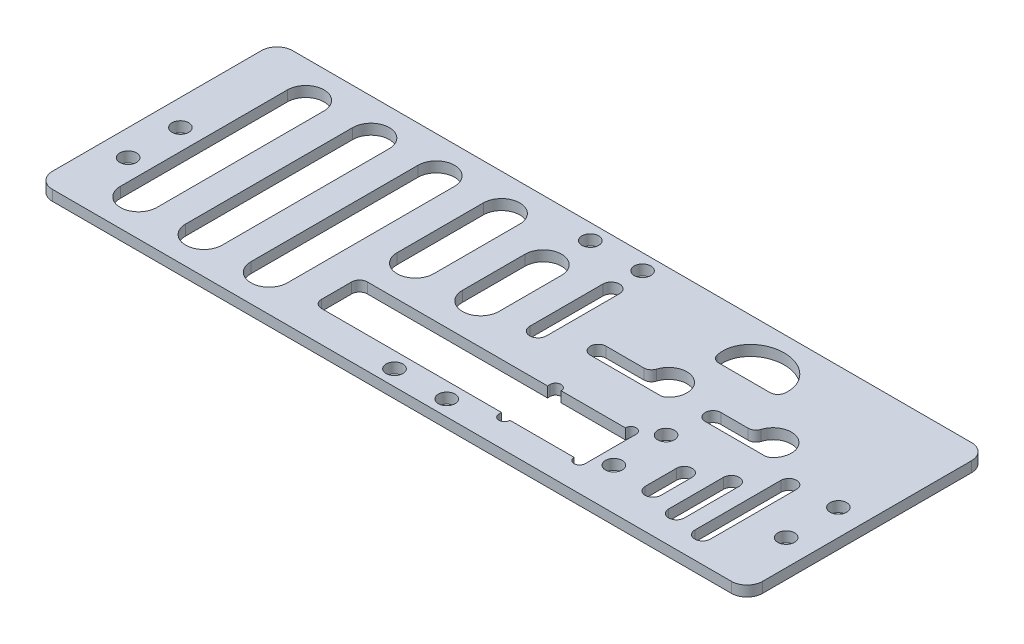
from build123d import *

# Parameters (mm, degrees)
SKETCH_1_W          = 136
SKETCH_1_H          = 46
SKETCH_1_R          = 1.6
EXTRUDE_1_DEPTH     = 2
CUT_EXTRUDE_1_DEPTH = 72.812255222
FILLET_R1_5_R       = 1.5
FILLET_R3_R         = 3


with BuildPart() as part:
    # 草图1 → 凸台-拉伸1 (new body)
    with BuildSketch(Plane(origin=(0, 0, 0), x_dir=(1, 0, 0), z_dir=(0, 1, 0))):
        Rectangle(SKETCH_1_W, SKETCH_1_H)
        with Locations(Location((-63, -0.5, 0), (0, 0, 270))):
            Circle(SKETCH_1_R, mode=Mode.SUBTRACT)
        with Locations(Location((-63, -10.5, 0), (0, 0, 270))):
            Circle(SKETCH_1_R, mode=Mode.SUBTRACT)
        with Locations(Location((-2.5, -20, 0), (0, 0, 270))):
            Circle(SKETCH_1_R, mode=Mode.SUBTRACT)
        with Locations(Location((7.5, -20, 0), (0, 0, 270))):
            Circle(SKETCH_1_R, mode=Mode.SUBTRACT)
        with Locations(Location((63, -10.5, 0), (0, 0, 90))):
            Circle(SKETCH_1_R, mode=Mode.SUBTRACT)
        with Locations(Location((63, -0.5, 0), (0, 0, 90))):
            Circle(SKETCH_1_R, mode=Mode.SUBTRACT)
        with Locations(Location((5, 20, 0), (0, 0, 270))):
            Circle(SKETCH_1_R, mode=Mode.SUBTRACT)
        with Locations(Location((-5, 20, 0), (0, 0, 270))):
            Circle(SKETCH_1_R, mode=Mode.SUBTRACT)
        with Locations(Location((34.5, -5, 0), (0, 0, 270))):
            Circle(SKETCH_1_R, mode=Mode.SUBTRACT)
        with Locations(Location((34.5, -15, 0), (0, 0, 270))):
            Circle(SKETCH_1_R, mode=Mode.SUBTRACT)
    extrude(amount=EXTRUDE_1_DEPTH)

    # 草图2 → 切除-拉伸1 (cut, through all)
    with BuildSketch(Plane(origin=(0, 2, 0), x_dir=(1, 0, 0), z_dir=(0, 1, 0))):
        with BuildLine():
            Line((-52, 16), (-52, -16))
            ThreePointArc((-52, -16), (-55.5, -19.5), (-59, -16))
            Line((-59, -16), (-59, 16))
            ThreePointArc((-59, 16), (-55.5, 19.5), (-52, 16))
        make_face()
        with BuildLine():
            Line((17.1, -7.7), (29.4, -7.7))
            ThreePointArc((29.4, -7.7), (30.45, -6.65), (31.5, -7.7))
            Line((31.5, -7.7), (31.5, -17.5))
            ThreePointArc((31.5, -17.5), (30.45, -18.55), (29.4, -17.5))
            Line((29.4, -17.5), (17.1, -17.5))
            ThreePointArc((17.1, -17.5), (16.05, -18.55), (15, -17.5))
            Line((15, -17.5), (15, -17))
            Line((15, -17), (-21, -17))
            Line((-21, -17), (-21, -8.2))
            Line((-21, -8.2), (15, -8.2))
            Line((15, -8.2), (15, -7.7))
            ThreePointArc((15, -7.7), (16.05, -6.65), (17.1, -7.7))
        make_face()
        with BuildLine():
            Line((-39.5, 16), (-39.5, -16))
            ThreePointArc((-39.5, -16), (-43, -19.5), (-46.5, -16))
            Line((-46.5, -16), (-46.5, 16))
            ThreePointArc((-46.5, 16), (-43, 19.5), (-39.5, 16))
        make_face()
        with BuildLine():
            Line((-27, 16), (-27, -16))
            ThreePointArc((-27, -16), (-30.5, -19.5), (-34, -16))
            Line((-34, -16), (-34, 16))
            ThreePointArc((-34, 16), (-30.5, 19.5), (-27, 16))
        make_face()
        with BuildLine():
            Line((-2, 11.5), (-2, -0.5))
            ThreePointArc((-2, -0.5), (-5.5, -4), (-9, -0.5))
            Line((-9, -0.5), (-9, 11.5))
            ThreePointArc((-9, 11.5), (-5.5, 15), (-2, 11.5))
        make_face()
        with BuildLine():
            Line((42.5, 4), (36, 4))
            ThreePointArc((36, 4), (34.5, 2.5), (36, 1))
            Line((36, 1), (47.802775638, 1))
            ThreePointArc((47.802775638, 1), (47.723410176, 7.046285831), (42.5, 4))
        make_face()
        with BuildLine():
            Line((41, -15.5), (41, -9.5))
            ThreePointArc((41, -9.5), (42.5, -8), (44, -9.5))
            Line((44, -9.5), (44, -15.5))
            ThreePointArc((44, -15.5), (42.5, -17), (41, -15.5))
        make_face()
        with BuildLine():
            Line((47, -17), (47, -6.5))
            ThreePointArc((47, -6.5), (48.5, -5), (50, -6.5))
            Line((50, -6.5), (50, -17))
            ThreePointArc((50, -17), (48.5, -18.5), (47, -17))
        make_face()
        with BuildLine():
            Line((53, -18), (53, -1.5))
            ThreePointArc((53, -1.5), (54.5, 0), (56, -1.5))
            Line((56, -1.5), (56, -18))
            ThreePointArc((56, -18), (54.5, -19.5), (53, -18))
        make_face()
        with BuildLine():
            Line((22.5, 4), (14, 4))
            ThreePointArc((14, 4), (12.5, 2.5), (14, 1))
            Line((14, 1), (27.802775638, 1))
            ThreePointArc((27.802775638, 1), (27.723410176, 7.046285831), (22.5, 4))
        make_face()
        with BuildLine():
            Line((38.555359619, 12), (26.555359619, 12))
            add(Edge.make_bspline(
                [(38.555359619, 12), (41.784518916, 19.940569638), (32.181153285, 19.940569638), (22.577787653, 19.940569638), (26.555359619, 12)],
                knots=[6.095299784, 6.095299784, 6.095299784, 8.050729179, 8.050729179, 10.006158574, 10.006158574, 10.006158574], degree=2, weights=[1, 0.558919028, 1, 0.558919028, 1]))
        make_face()
        with BuildLine():
            Line((3.4, 0), (3.4, 14))
            ThreePointArc((3.4, 14), (5, 15.6), (6.6, 14))
            Line((6.6, 14), (6.6, 0))
            ThreePointArc((6.6, 0), (5, -1.6), (3.4, 0))
        make_face()
        with BuildLine():
            Line((-21.5, -0.5), (-21.5, 16))
            ThreePointArc((-21.5, 16), (-18, 19.5), (-14.5, 16))
            Line((-14.5, 16), (-14.5, -0.5))
            ThreePointArc((-14.5, -0.5), (-18, -4), (-21.5, -0.5))
        make_face()
    extrude(amount=-CUT_EXTRUDE_1_DEPTH, mode=Mode.SUBTRACT)

    # R1.5 镂空圆角
    fillet_r1_5_edges = [part.edges().sort_by_distance(p)[0] for p in [
        (-21, 1, 8.2),
        (-21, 1, 17),
        (38.555359619, 1, -12),
        (26.555359619, 1, -12),
        (22.5, 1, -4),
        (27.802775638, 1, -1),
        (42.5, 1, -4),
        (47.802775638, 1, -1),
    ]]
    fillet(fillet_r1_5_edges, radius=FILLET_R1_5_R)

    # R3 外缘圆角
    fillet_r3_edges = [part.edges().sort_by_distance(p)[0] for p in [
        (-68, 1, -23),
        (68, 1, -23),
        (68, 1, 23),
        (-68, 1, 23),
    ]]
    fillet(fillet_r3_edges, radius=FILLET_R3_R)


solid = part.part
